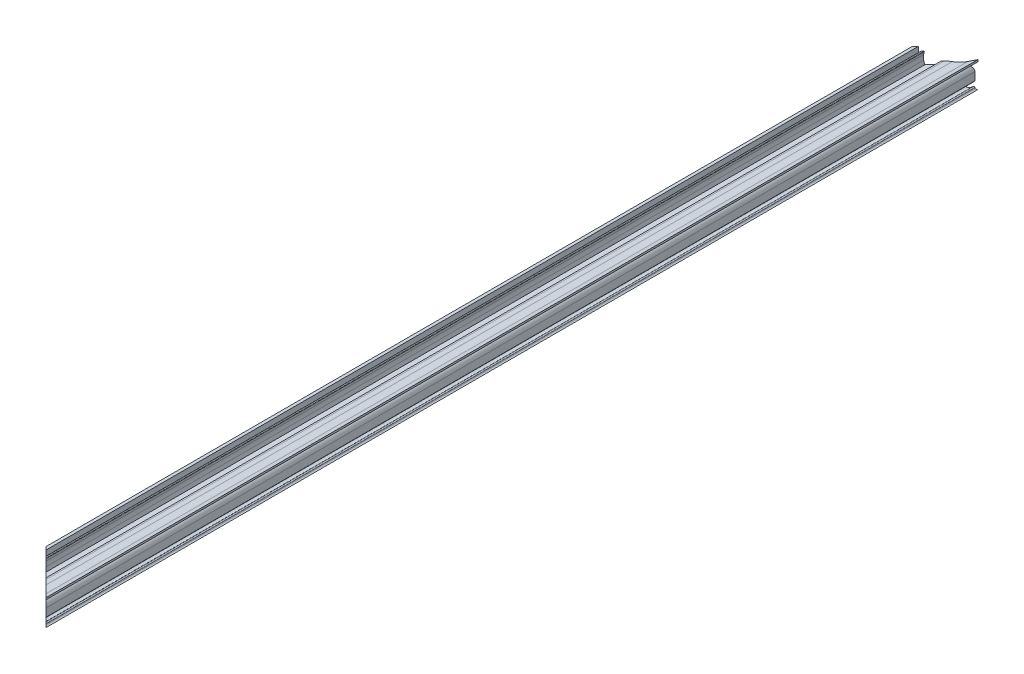
from build123d import *

# Parameters (mm, degrees)
EXTRUDE1_DEPTH = 624
EXTRUDE2_DEPTH = 30


with BuildPart() as part:
    # Sketch2 → Extrude1 (new body)
    with BuildSketch(Plane.XY):
        with BuildLine():
            Line((27.429618111, 61.203514875), (27.429618111, 62.483514875))
            Line((27.429618111, 62.483514875), (27.063725093, 65.097036429))
            ThreePointArc((27.063725093, 65.097036429), (26.9381678, 66.899458408), (27.063725093, 68.701880387))
            Line((27.063725093, 68.701880387), (27.290970266, 70.325060195))
            ThreePointArc((27.290970266, 70.325060195), (27.40740123, 70.522960701), (27.629667144, 70.580568366))
            Line((27.629667144, 70.580568366), (28.223872192, 70.497379659))
            ThreePointArc((28.223872192, 70.497379659), (28.421772697, 70.380948695), (28.479380362, 70.158682782))
            Line((28.479380362, 70.158682782), (28.252135189, 68.535502974))
            ThreePointArc((28.252135189, 68.535502974), (28.1381678, 66.899458408), (28.252135189, 65.263413843))
            Line((28.252135189, 65.263413843), (28.629618111, 62.56710726))
            Line((28.629618111, 62.56710726), (34.119618111, 62.56710726))
            Line((34.119618111, 62.56710726), (34.119618111, 64.76710726))
            Line((34.119618111, 64.76710726), (35.119618111, 64.76710726))
            ThreePointArc((35.119618111, 64.76710726), (36.498022986, 64.671651671), (37.850112572, 64.38710726))
            ThreePointArc((37.850112572, 64.38710726), (40.451975855, 64.047973934), (43.040517634, 64.47710726))
            Line((43.040517634, 64.47710726), (46.429618111, 65.567355231))
            Line((46.429618111, 65.567355231), (46.429618111, 64.306791917))
            Line((46.429618111, 64.306791917), (43.408001834, 63.334760831))
            ThreePointArc((43.408001834, 63.334760831), (40.472780352, 62.848154292), (37.522453236, 63.23270726))
            ThreePointArc((37.522453236, 63.23270726), (36.431587911, 63.468758554), (35.319618111, 63.564834239))
            Line((35.319618111, 63.564834239), (35.319618111, 62.56710726))
            Line((35.319618111, 62.56710726), (41.399618111, 62.56710726))
            ThreePointArc((41.399618111, 62.56710726), (44.228045236, 61.395534384), (45.399618111, 58.56710726))
            Line((45.399618111, 58.56710726), (45.399618111, 53.252873744))
            ThreePointArc((45.399618111, 53.252873744), (45.127835843, 52.807995483), (44.607951444, 52.846757313))
            ThreePointArc((44.607951444, 52.846757313), (41.599927405, 51.269233396), (44.662909839, 49.801265776))
            ThreePointArc((44.662909839, 49.801265776), (45.204517239, 49.836690545), (45.440067721, 49.347702344))
            ThreePointArc((45.440067721, 49.347702344), (45.673249329, 48.549369428), (46.429618111, 48.203514875))
            Line((46.429618111, 48.203514875), (24.429618111, 48.203514875))
            Line((24.429618111, 48.203514875), (24.429618111, 73.203514875))
            Line((24.429618111, 73.203514875), (26.429618111, 73.203514875))
            Line((26.429618111, 73.203514875), (26.429618111, 61.203514875))
            Line((26.429618111, 61.203514875), (27.429618111, 61.203514875))
        make_face()
    extrude(amount=EXTRUDE1_DEPTH)

    # Sketch3 → Extrude2 (cut)
    with BuildSketch(Plane.XZ.offset(-48.203514875)):
        Polygon((46.429618111, 624), (24.429618111, 624), (24.429618111, 602), align=None)
        Polygon((46.429618111, 0), (24.429618111, 0), (24.429618111, 22), align=None)
    extrude(amount=-EXTRUDE2_DEPTH, mode=Mode.SUBTRACT)


solid = part.part
